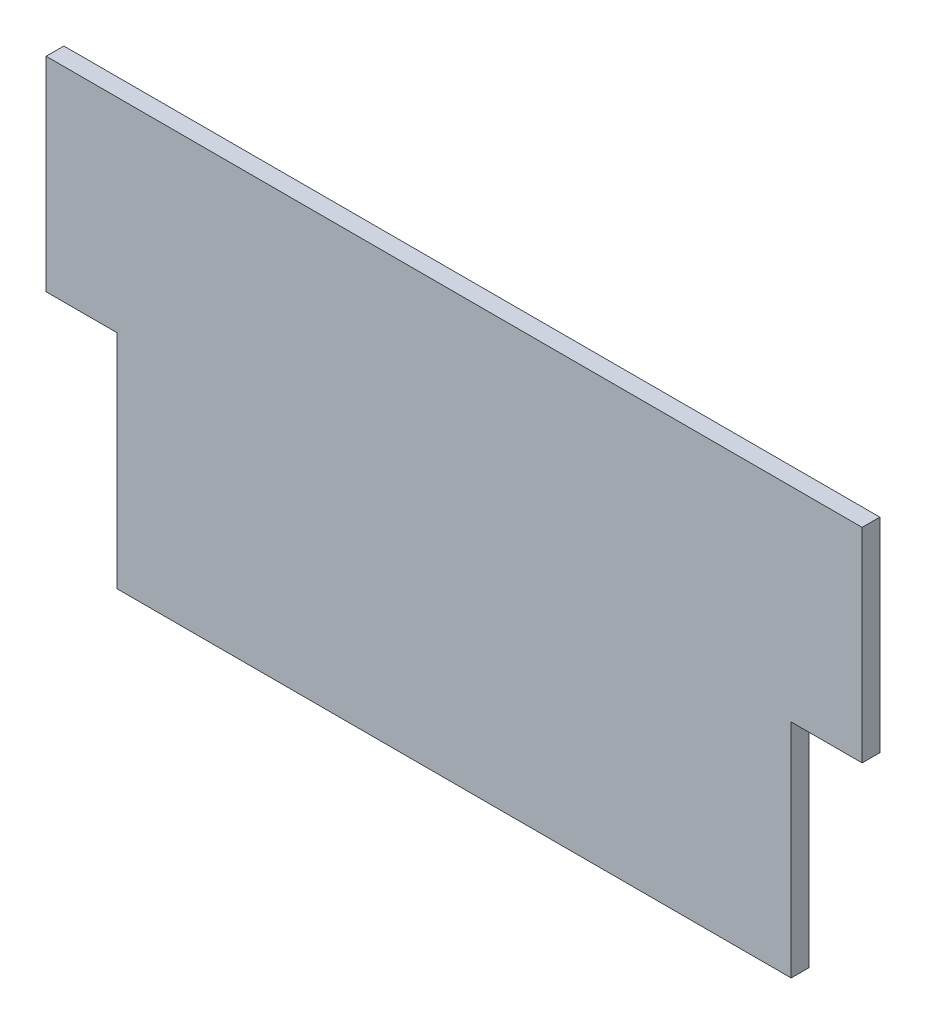
SolidWorks part; units mm, degrees
ref_plane "前视基准面" through (0, 0, 0) normal (0, 0, 1) x (1, 0, 0)
ref_plane "上视基准面" through (0, 0, 0) normal (0, 1, 0) x (1, 0, 0)
ref_plane "右视基准面" through (0, 0, 0) normal (1, 0, 0) x (0, 0, -1)
sketch "草图1" plane through (0, 0, 0) normal (0, 0, 1) x (1, 0, 0)
  line L0 (0, 0) -> (460, 0)
  line L1 (460, 0) -> (460, -115)
  line L2 (0, 0) -> (0, -115)
  line L3 (0, -115) -> (50, -115)
  line L4 (460, -115) -> (410, -115)
  line L5 (410, -115) -> (410, -240)
  line L6 (410, -240) -> (50, -240)
  line L7 (50, -240) -> (50, -115)
extrude "凸台-拉伸1" add sketch "草图1" along normal blind 10
sketch "草图2" plane through (410, 0, 0) normal (1, 0, 0) x (0, 0, -1)
  line L8 (0, -240) -> (0, -115)
  line L9 (0, -115) -> (-10, -115)
  line L10 (-10, -115) -> (-10, -240)
  line L11 (-10, -240) -> (0, -240)
  line L12 (0, -240) -> (0, -115)
  line L13 (0, -115) -> (-10, -115)
  line L14 (-10, -115) -> (-10, -240)
  line L15 (-10, -240) -> (0, -240)
  dimension "D1" = 0
extrude "凸台-拉伸2" add sketch "草图2" along normal blind 10
sketch "草图3" plane through (50, 0, 0) normal (-1, 0, 0) x (0, 0, 1)
  line L8 (0, -115) -> (0, -240)
  line L9 (0, -240) -> (10, -240)
  line L10 (10, -240) -> (10, -115)
  line L11 (10, -115) -> (0, -115)
  line L12 (0, -115) -> (0, -240)
  line L13 (0, -240) -> (10, -240)
  line L14 (10, -240) -> (10, -115)
  line L15 (10, -115) -> (0, -115)
  dimension "D1" = 0
extrude "凸台-拉伸3" add sketch "草图3" along normal blind 10
sketch "草图4" plane through (0, 0, 0) normal (0, 1, 0) x (1, 0, 0)
  line L0 (230, 0) -> (230, -10)
  line L1 (460, 0) -> (0, 0) construction
  line L2 (460, -10) -> (0, -10) construction
sketch "草图5" plane through (0, 0, 10) normal (0, 0, 1) x (1, 0, 0)
  line L0 (230, 0) -> (230, -5.6598)
  line L1 (460, 0) -> (0, 0) construction
  line L2 (230, -5.6598) -> (230, -11.8788)
